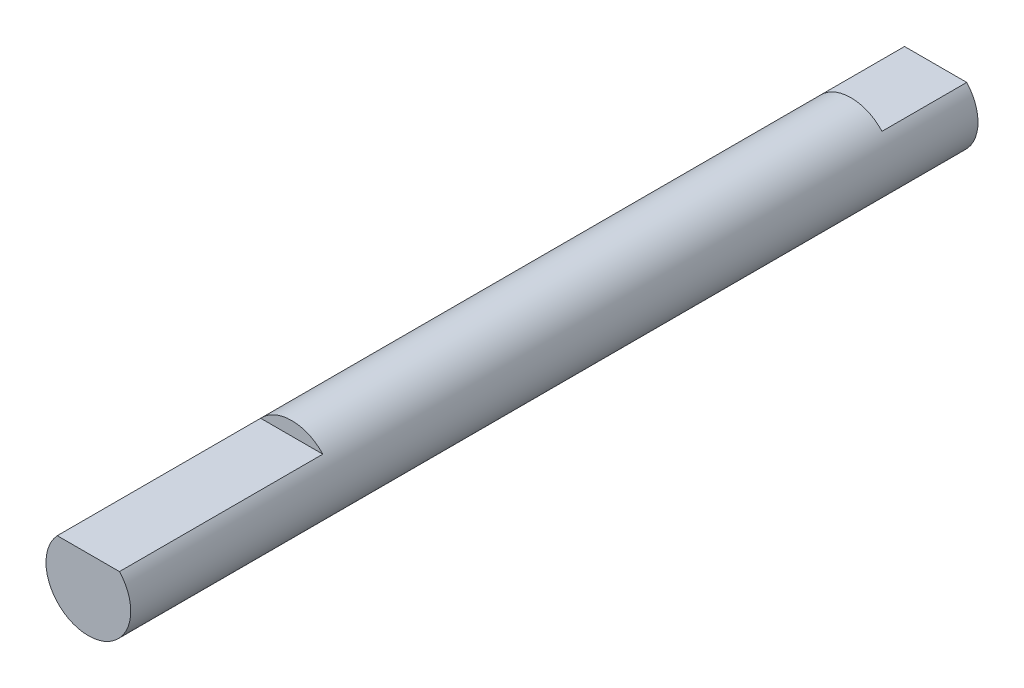
from build123d import *

# Parameters (mm, degrees)
SKETCH1_R           = 2.5
BOSS_EXTRUDE1_DEPTH = 50
CUT_EXTRUDE1_DEPTH  = 5
CUT_EXTRUDE3_START  = -12
CUT_EXTRUDE3_DEPTH  = 12


with BuildPart() as part:
    # Sketch1 → Boss-Extrude1 (new body)
    with BuildSketch(Plane.XY):
        Circle(SKETCH1_R)
    extrude(amount=BOSS_EXTRUDE1_DEPTH)

    # Sketch2 → Cut-Extrude1 (cut)
    with BuildSketch(Plane(origin=(0, 0, 0), x_dir=(-1, 0, 0), z_dir=(0, 0, -1))):
        with BuildLine():
            Line((-1.835, 1.69787367), (1.835, 1.69787367))
            ThreePointArc((1.835, 1.69787367), (0, 2.5), (-1.835, 1.69787367))
        make_face()
    extrude(amount=-CUT_EXTRUDE1_DEPTH, mode=Mode.SUBTRACT)

    # Sketch3 → Cut-Extrude3 (cut)
    with BuildSketch(Plane.XY.offset(50).offset(CUT_EXTRUDE3_START)):
        with BuildLine():
            Line((-1.835, 1.69787367), (1.835, 1.69787367))
            ThreePointArc((1.835, 1.69787367), (0, 2.5), (-1.835, 1.69787367))
        make_face()
    extrude(amount=CUT_EXTRUDE3_DEPTH, mode=Mode.SUBTRACT)


solid = part.part
